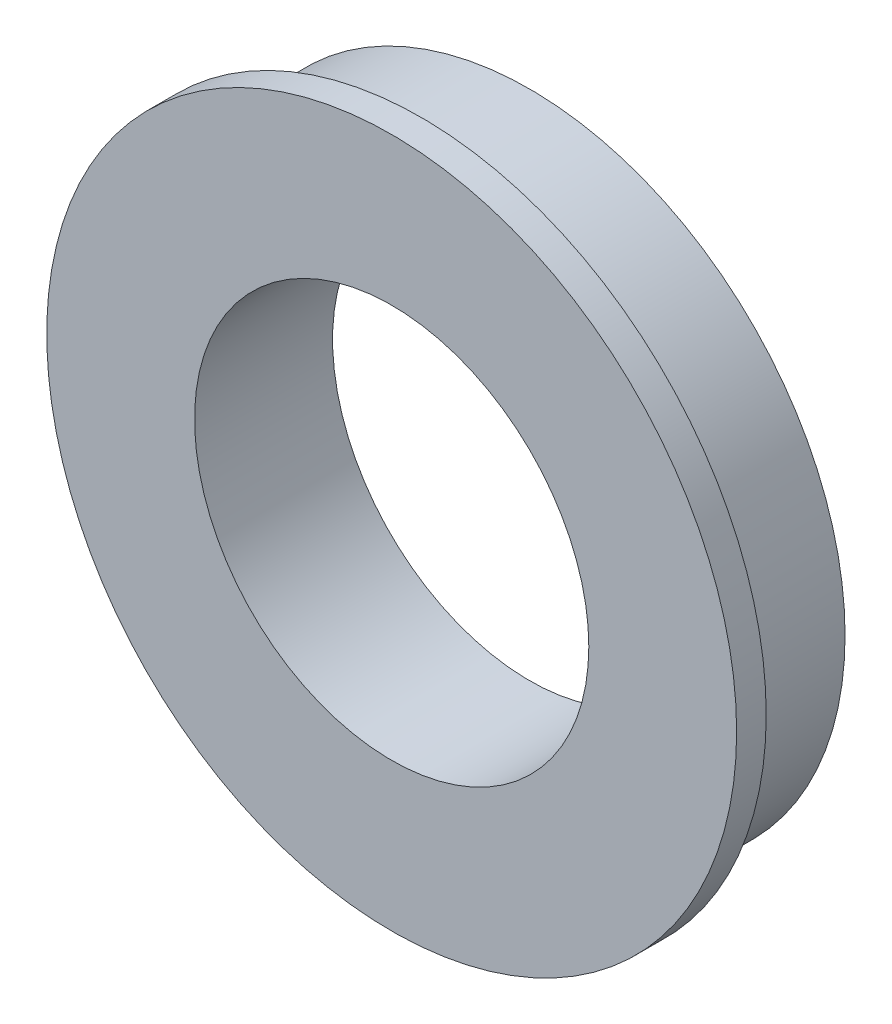
SolidWorks part; units mm, degrees
material "镀铬不锈钢"
ref_plane "前视基准面" through (0, 0, 0) normal (0, 0, 1) x (1, 0, 0)
ref_plane "上视基准面" through (0, 0, 0) normal (0, 1, 0) x (1, 0, 0)
ref_plane "右视基准面" through (0, 0, 0) normal (1, 0, 0) x (0, 0, -1)
other "Configuration Table"
sketch "草图1" plane through (0, 0, 0) normal (0, 0, 1) x (1, 0, 0)
  circle A0 centre (0, 0) radius 10
  circle A1 centre (0, 0) radius 16
  dimension "D1" = 20
  dimension "D2" = 32
extrude "凸台-拉伸1" add sketch "草图1" along normal blind 7
sketch "草图2" plane through (0, 0, 7) normal (0, 0, 1) x (1, 0, 0)
  circle A0 centre (0, 0) radius 17.5
  circle A1 centre (0, 0) radius 16 construction
  circle A2 centre (0, 0) radius 16
  dimension "D1" = 35
extrude "凸台-拉伸2" add sketch "草图2" against normal blind 1.5
